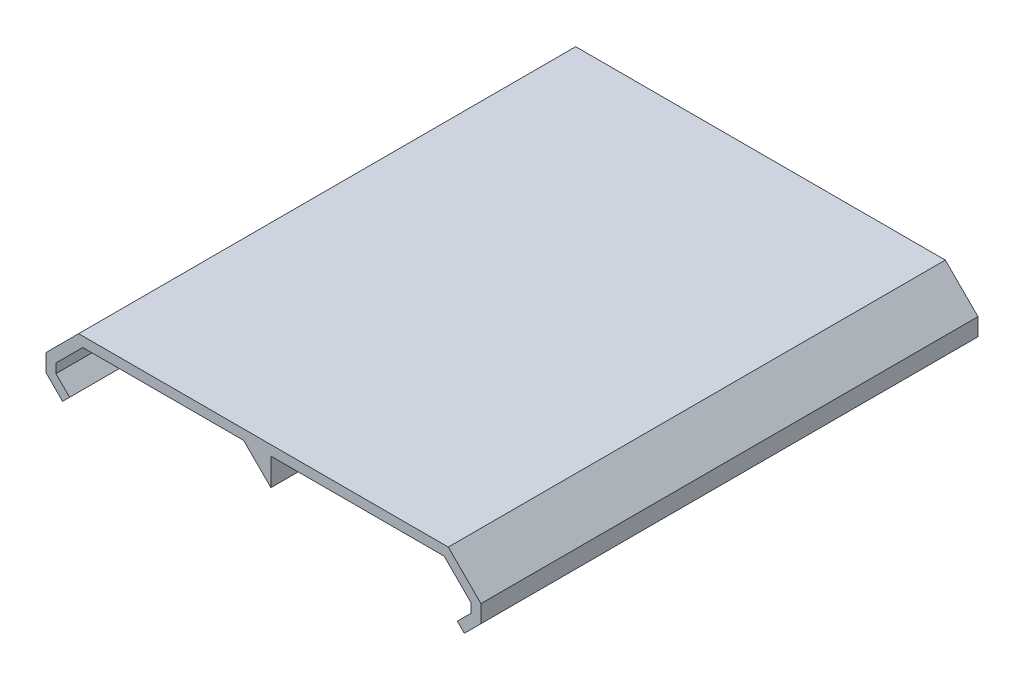
from build123d import *

# Parameters (mm, degrees)
EXTRUDE_THIN1_DEPTH = 200
BOSS_EXTRUDE1_DEPTH = 37


with BuildPart() as part:
    # Sketch1 → Extrude-Thin1 (new body)
    with BuildSketch(Plane.XY):
        Polygon((78, 32), (83.5, 37.5), (83.5, 41.207106781), (72.707106781, 52), (-72.707106781, 52), (-83.5, 41.207106781), (-83.5, 37.5), (-78, 32), (-80.828427125, 29.171572875), (-87.5, 35.843145751), (-87.5, 42.863961031), (-74.363961031, 56), (74.363961031, 56), (87.5, 42.863961031), (87.5, 35.843145751), (80.828427125, 29.171572875), align=None)
    extrude(amount=-EXTRUDE_THIN1_DEPTH)

    # Sketch2 → Boss-Extrude1 (add)
    with BuildSketch(Plane.XY):
        Polygon((-7.989949494, 52), (3, 52), (3, 41.010050506), align=None)
    extrude(amount=-BOSS_EXTRUDE1_DEPTH)


solid = part.part
